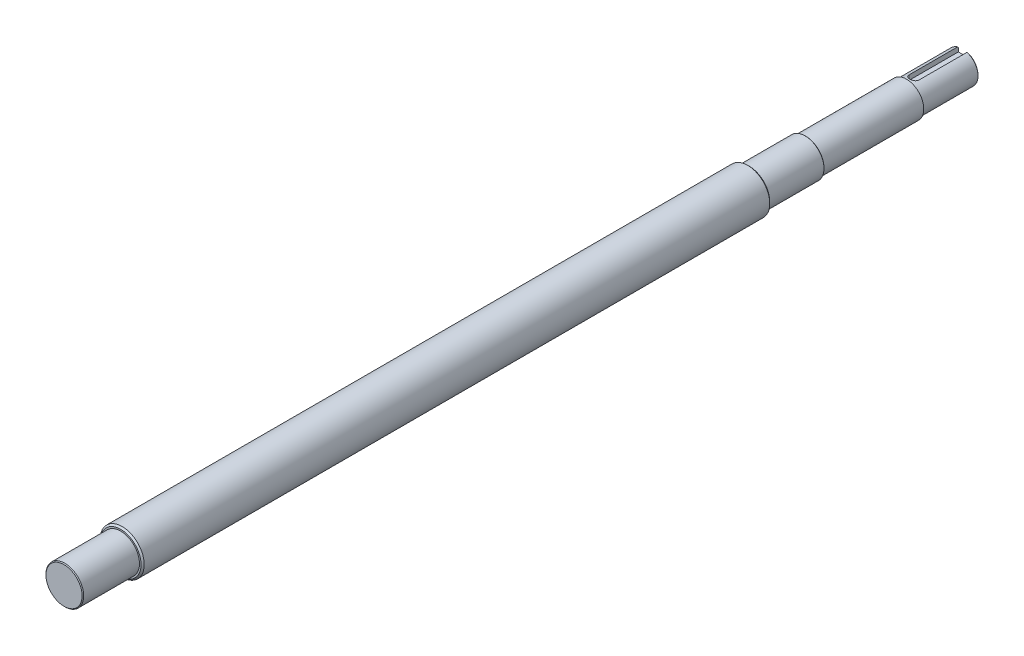
SolidWorks part; units mm, degrees
ref_plane "Front Plane" through (0, 0, 0) normal (0, 0, 1) x (1, 0, 0)
ref_plane "Top Plane" through (0, 0, 0) normal (0, 1, 0) x (1, 0, 0)
ref_plane "Right Plane" through (0, 0, 0) normal (1, 0, 0) x (0, 0, -1)
sketch "Sketch1" plane through (0, 0, 0) normal (0, 0, 1) x (1, 0, 0)
  circle A0 centre (0, 0) radius 12
extrude "Boss-Extrude1" add sketch "Sketch1" against normal up to surface (472 mm away)
sketch "Sketch2" plane through (0, 0, -472) normal (0, 0, -1) x (-1, 0, 0)
  circle A0 centre (0, 0) radius 11
  dimension "D1" = 22
extrude "Boss-Extrude2" add sketch "Sketch2" along normal blind 100
ref_plane "Plane1" through (0, 0, -36) normal (0, 0, 1) x (1, 0, 0)
sketch "Sketch4" plane through (0, 0, -36) normal (0, 0, 1) x (1, 0, 0)
  circle A0 centre (0, 0) radius 14
  dimension "D1" = 28
extrude "Boss-Extrude3" add sketch "Sketch4" against normal blind 400
cosmetic thread "Cosmetic Thread1" parameters "D2"=27
chamfer "Chamfer1" distance 1 angle 45 2 edges at (14, 0, -436) (14, 0, -36)
chamfer "Chamfer2" distance 0.5 angle 45 1 edges at (12, 0, 0)
chamfer "Chamfer3" distance 0.5 angle 45 1 edges at (0, 12, -472)
sketch "Sketch5" plane through (0, 0, -572) normal (0, 0, -1) x (-1, 0, 0)
  circle A0 centre (0, 0) radius 10
  circle A1 centre (0, 0) radius 20
  dimension "D1" = 20
  dimension "D2" = 40
extrude "Cut-Extrude1" cut sketch "Sketch5" against normal blind 36
ref_plane "Plane2" through (0, 6.5, 0) normal (0, 1, 0) x (1, 0, 0)
sketch "Sketch6" plane through (0, 6.5, 0) normal (0, 1, 0) x (1, 0, 0)
  line L0 (0, 536) -> (0, 593.3081) construction
  line L1 (11, 536) -> (-11, 536) construction
  line L2 (0, 576.6485) -> (0, 541) construction
  line L3 (3, 576.6485) -> (3, 541)
  line L4 (-3, 576.6485) -> (-3, 541)
  arc A0 (3, 576.6485) -> (-3, 576.6485) centre (0, 576.6485) ccw
  arc A1 (-3, 541) -> (3, 541) centre (0, 541) ccw
  point P7 (0, 558.8242)
  dimension "D2" = 5
  dimension "D1" = 6
extrude "Cut-Extrude2" cut sketch "Sketch6" along normal through all
chamfer "Chamfer4" distance 0.5 angle 45 1 edges at (0, -10, -572)
